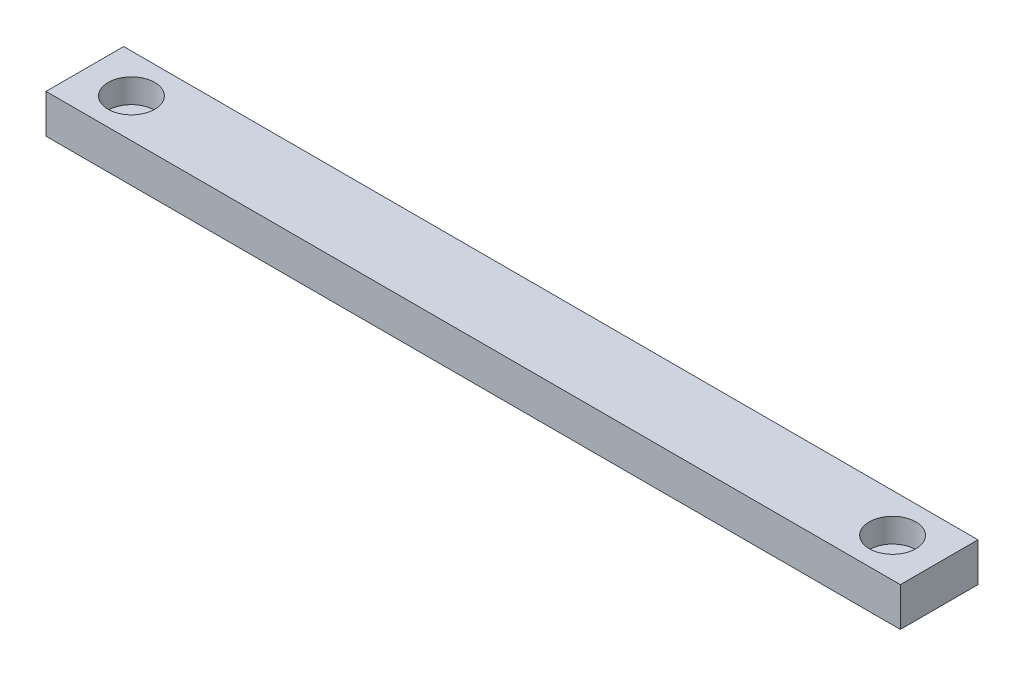
SolidWorks part; units mm, degrees
ref_plane "Front Plane" through (0, 0, 0) normal (0, 0, 1) x (1, 0, 0)
ref_plane "Top Plane" through (0, 0, 0) normal (0, 1, 0) x (1, 0, 0)
ref_plane "Right Plane" through (0, 0, 0) normal (1, 0, 0) x (0, 0, -1)
other "Configuration Table"
sketch "Sketch1" plane through (0, 0, 0) normal (0, 1, 0) x (1, 0, 0)
  line L1 (-55, 5) -> (55, 5)
  line L2 (-55, 5) -> (-55, -5)
  line L3 (-55, -5) -> (55, -5)
  line L4 (55, 5) -> (55, -5)
  line L5 (-55, 5) -> (55, -5) construction
  line L6 (-55, -5) -> (55, 5) construction
  point P0 (0, 0)
  dimension "D1" = 110
  dimension "D2" = 10
extrude "Boss-Extrude1" add sketch "Sketch1" along normal blind 5
sketch "Sketch2" plane through (0, 5, 0) normal (0, 1, 0) x (1, 0, 0)
  line L0 (-55, 5) -> (-55, -5) construction
  line L1 (55, -5) -> (55, 5) construction
  circle A0 centre (-49, 0) radius 3
  circle A1 centre (49, 0) radius 3
  point P8 (-55, 0)
  dimension "D1" = 6
  dimension "D3" = 6
  dimension "D2" = 6
  dimension "D4" = 6
extrude "Cut-Extrude1" cut sketch "Sketch2" against normal blind 3.1
